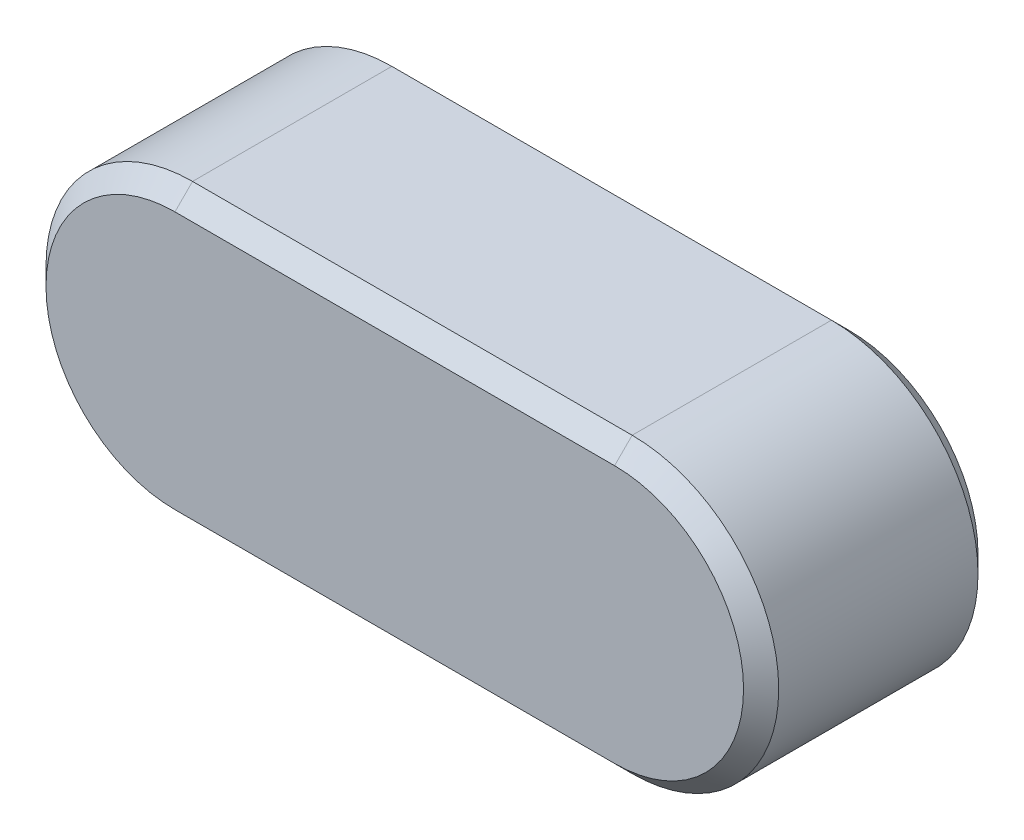
from build123d import *

# Parameters (mm, degrees)
BASEKEY_DEPTH = 4
CHAMFER1_SIZE = 0.6


with BuildPart() as part:
    # Sketch1 → BaseKey (new, symmetric)
    with BuildSketch(Plane.XY):
        with BuildLine():
            Line((-15, 5), (0, 5))
            ThreePointArc((0, 5), (5, 0), (0, -5))
            Line((0, -5), (-15, -5))
            ThreePointArc((-15, -5), (-20, 0), (-15, 5))
        make_face()
    extrude(amount=BASEKEY_DEPTH, both=True)

    # Chamfer1
    chamfer1_edges = [part.edges().sort_by_distance(p)[0] for p in [
        (5, 0, 4),
        (-7.5, 5, 4),
        (-20, 0, 4),
        (-7.5, 5, -4),
        (5, 0, -4),
        (-7.5, -5, -4),
        (-20, 0, -4),
        (-7.5, -5, 4),
    ]]
    chamfer(chamfer1_edges, length=CHAMFER1_SIZE)


solid = part.part
